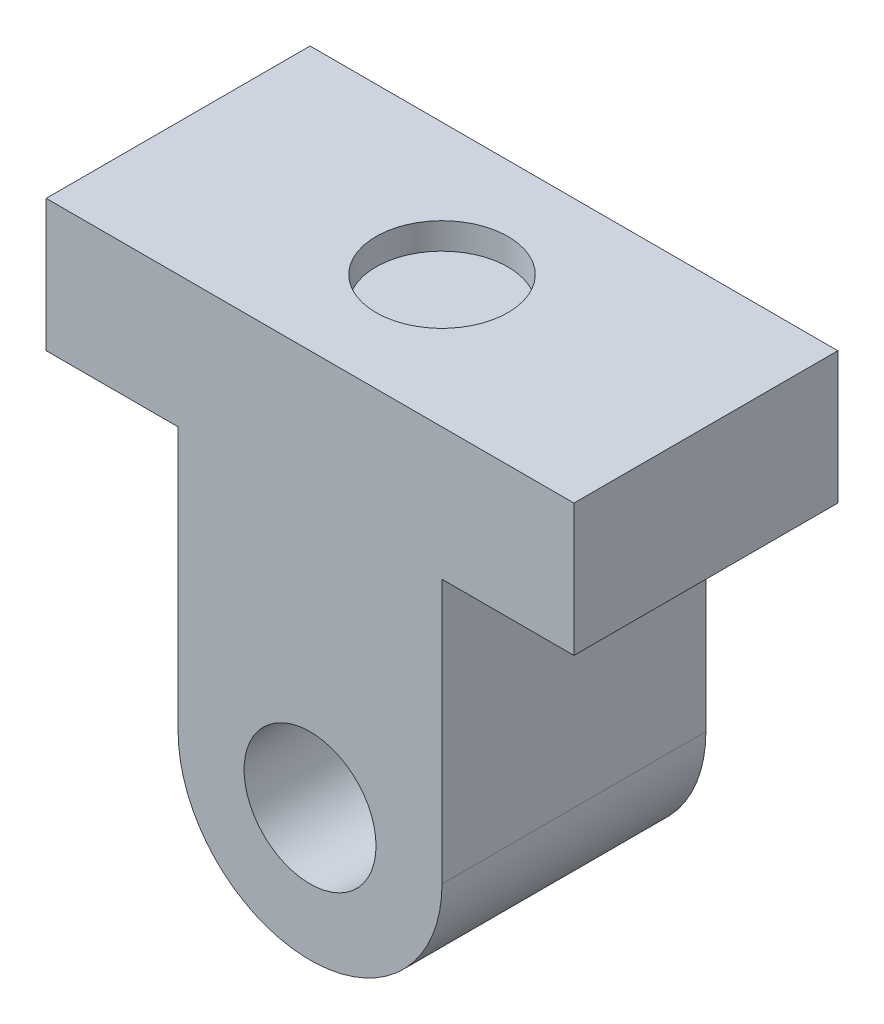
from build123d import *

# Parameters (mm, degrees)
SKETCH1_R           = 2.5
BOSS_EXTRUDE1_DEPTH = 10
SKETCH2_R           = 2.5
CUT_EXTRUDE1_DEPTH  = 1


with BuildPart() as part:
    # Sketch1 → Boss-Extrude1 (new body)
    with BuildSketch(Plane.XY):
        with BuildLine():
            Line((-5, 0), (-5, 10))
            Line((-5, 10), (-10, 10))
            Line((-10, 10), (-10, 15))
            Line((-10, 15), (10, 15))
            Line((10, 15), (10, 10))
            Line((10, 10), (5, 10))
            Line((5, 10), (5, 0))
            ThreePointArc((5, 0), (0, -5), (-5, 0))
        make_face()
        Circle(SKETCH1_R, mode=Mode.SUBTRACT)
    extrude(amount=BOSS_EXTRUDE1_DEPTH)

    # Sketch2 → Cut-Extrude1 (cut)
    with BuildSketch(Plane(origin=(0, 15, 0), x_dir=(1, 0, 0), z_dir=(0, 1, 0))):
        with Locations(Location((0, -5, 0), (0, 0, 270))):
            Circle(SKETCH2_R)
    extrude(amount=-CUT_EXTRUDE1_DEPTH, mode=Mode.SUBTRACT)


solid = part.part
